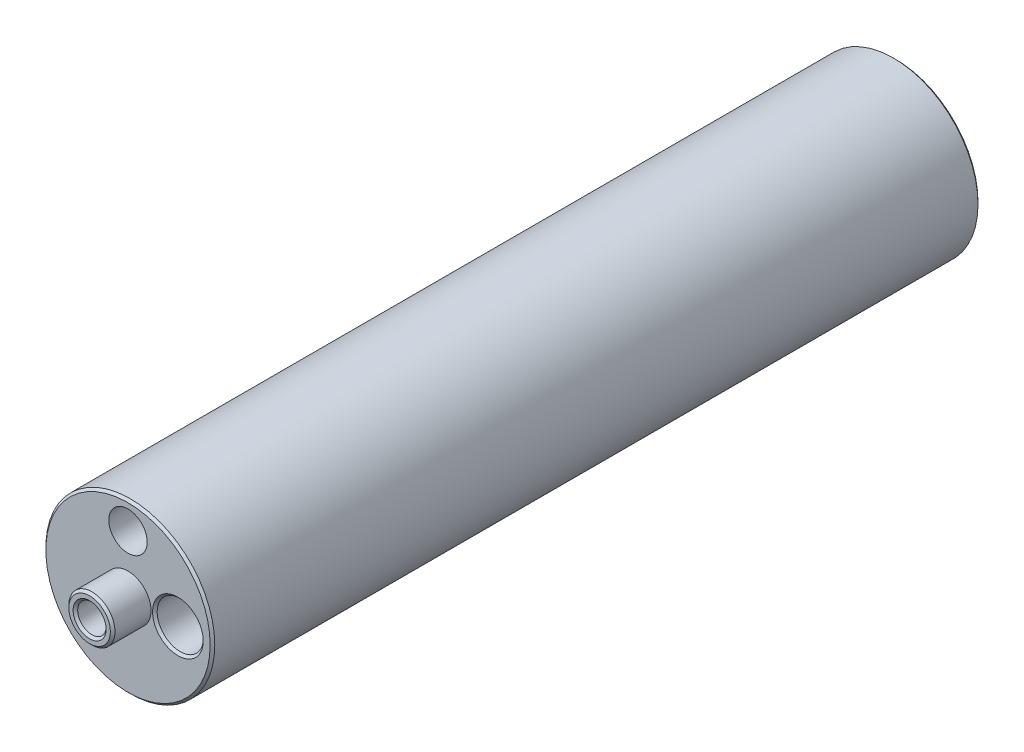
from build123d import *

# Parameters (mm, degrees)
SKETCH1_R             = 11
BOSS_EXTRUDE1_DEPTH   = 100
SKETCH2_R             = 3
BOSS_EXTRUDE2_DEPTH   = 5
SKETCH3_R             = 1.85
CUT_EXTRUDE1_DEPTH    = 107.146125695
SKETCH4_R             = 3
CUT_EXTRUDE2_DEPTH    = 102.202766761
M6_TAPPED_HOLE1_D     = 5
M6_TAPPED_HOLE1_DEPTH = 10
M6_TAPPED_HOLE1_TIP   = 1.502151548
CHAMFER1_SIZE         = 0.3


with BuildPart() as part:
    # Sketch1 → Boss-Extrude1 (new body)
    with BuildSketch(Plane.XY):
        Circle(SKETCH1_R)
    extrude(amount=BOSS_EXTRUDE1_DEPTH)

    # Sketch2 → Boss-Extrude2 (add)
    with BuildSketch(Plane.XY.offset(100)):
        Circle(SKETCH2_R)
    extrude(amount=BOSS_EXTRUDE2_DEPTH)

    # Sketch3 → Cut-Extrude1 (cut, through all)
    with BuildSketch(Plane.XY.offset(105)):
        Circle(SKETCH3_R)
    extrude(amount=-CUT_EXTRUDE1_DEPTH, mode=Mode.SUBTRACT)

    # Sketch4 → Cut-Extrude2 (cut, through all)
    with BuildSketch(Plane.XY.offset(100)):
        with Locations((6.5, 0)):
            Circle(SKETCH4_R)
    extrude(amount=-CUT_EXTRUDE2_DEPTH, mode=Mode.SUBTRACT)

    # M6 Tapped Hole1
    with Locations(Plane.XY.offset(100)):
        with Locations((0, 7.5)):
            Hole(M6_TAPPED_HOLE1_D / 2, depth=M6_TAPPED_HOLE1_DEPTH)
            with Locations((0, 0, -(M6_TAPPED_HOLE1_DEPTH + M6_TAPPED_HOLE1_TIP / 2))):  # 118° drill point
                Cone(0, M6_TAPPED_HOLE1_D / 2, M6_TAPPED_HOLE1_TIP, mode=Mode.SUBTRACT)

    # Chamfer1
    chamfer1_edges = [part.edges().sort_by_distance(p)[0] for p in [
        (-1.85, 0, 0),
        (-1.85, 0, 105),
        (3.5, 0, 0),
        (3.5, 0, 100),
        (-11, 0, 0),
        (-11, 0, 100),
        (-3, 0, 105),
    ]]
    chamfer(chamfer1_edges, length=CHAMFER1_SIZE)


solid = part.part
